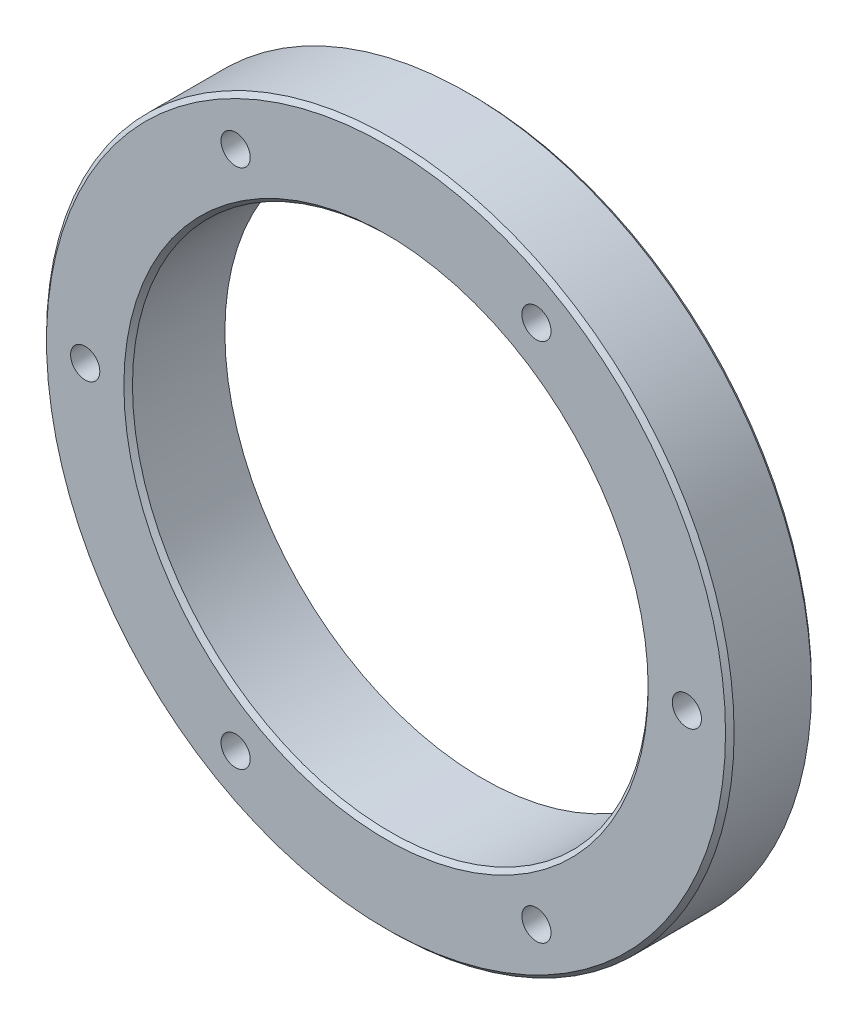
SolidWorks part; units mm, degrees
ref_plane "Front Plane" through (0, 0, 0) normal (0, 0, 1) x (1, 0, 0)
ref_plane "Top Plane" through (0, 0, 0) normal (0, 1, 0) x (1, 0, 0)
ref_plane "Right Plane" through (0, 0, 0) normal (1, 0, 0) x (0, 0, -1)
sketch "Sketch1" plane through (0, 0, 0) normal (0, 0, 1) x (1, 0, 0)
  circle A0 centre (0, 0) radius 80
  circle A1 centre (0, 0) radius 60
extrude "Boss-Extrude1" add sketch "Sketch1" along normal blind 20
sketch "Sketch2" plane through (0, 0, 20) normal (0, 0, 1) x (1, 0, 0)
  circle A2 centre (35, 60.6218) radius 3.5
  circle A4 centre (70, 0) radius 3.5
  circle A6 centre (35, -60.6218) radius 3.5
  circle A8 centre (-35, -60.6218) radius 3.5
  circle A10 centre (-70, 0) radius 3.5
  circle A12 centre (-35, 60.6218) radius 3.5
  point P29 (0, 0)
hole_wizard "M8x1.25 Tapped Hole2" positions "3DSketch1" profile "Sketch5" tap size "M8x1.25" standard "Ansi Metric"
sketch3d "3DSketch1"
  point P0 (-35, 60.6218, 20)
  point P3 (-70, 0, 20)
  point P6 (-35, -60.6218, 20)
  point P9 (35, -60.6218, 20)
  point P12 (70, 0, 20)
  point P15 (35, 60.6218, 20)
sketch "Sketch5" plane through (-35, 60.6218, 20) normal (1, 0, 0) x (0, -1, 0)
  line L0 (0, 0) -> (0, 20.0429)
  line L1 (0, 20.0429) -> (3.4, 18)
  line L2 (3.4, 18) -> (3.4, 0)
  line L5 (3.4, 0) -> (0, 0)
  line L10 (0, 20.0429) -> (-3.4, 18) construction
  line L11 (0, -6.35) -> (0, 107.95) construction
  dimension "螺纹孔钻头直径" = 6.8
  dimension "螺纹孔钻头深度" = 18
  dimension "导头角度" = 118
cosmetic thread "Cosmetic thread 2" parameters "D1"=10, "D2"=8
cosmetic thread "Cosmetic thread 3" parameters "D1"=10, "D2"=8
cosmetic thread "Cosmetic thread 4" parameters "D1"=10, "D2"=8
cosmetic thread "Cosmetic thread 5" parameters "D1"=10, "D2"=8
cosmetic thread "Cosmetic thread 6" parameters "D1"=10, "D2"=8
cosmetic thread "Cosmetic thread 7" parameters "D1"=10, "D2"=8
chamfer "Chamfer1" distance 1 angle 45 3 edges at (80, 0, 20) (80, 0, 0) (60, 0, 20)
sketch "Sketch6" plane through (0, 0, 0) normal (0, 0, -1) x (-1, 0, 0)
  circle A0 centre (0, 0) radius 60
  circle A1 centre (0, 0) radius 75
extrude "Boss-Extrude2" add sketch "Sketch6" along normal blind 2.5
